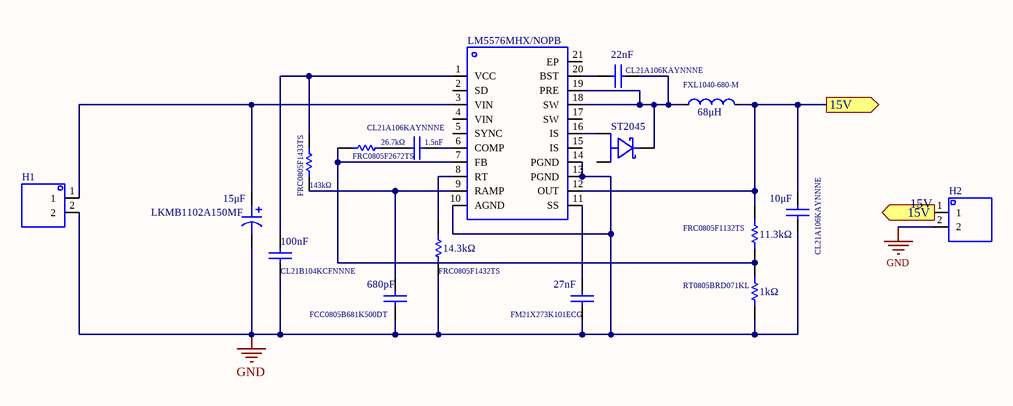
[diagram p0: MISC51833-3.schdoc]
# Altium project MISC51833-2.PrjPcb
1 sheet, 17 parts. Net scope: flat (ports and power ports of the same name join across sheets).
Board file: MISC51833.pcbdoc

## Sheet MISC51833-3.schdoc
size 292 x 193 mm; Name: MISC51833

### Parts
15μF  LKMB1102A150MF  [CAP-TH_BD5.0-P2.00-D0.8-FD]
C1  CL21A106KAYNNNE  value 1.5nF  [C0805]
C2  CL21A106KAYNNNE  value 22nF  [C0805]
C3  CL21A106KAYNNNE  value 10μF  [C0805]
C4  FCC0805B681K500DT  value 680pF  [C0805]
C5  FM21X273K101ECG  value 27nF  [C0805]
FRC0805F1132TS  value 11.3kΩ  [R0805]
FRC0805F1432TS  value 14.3kΩ  [R0805]
FRC0805F1433TS  value 143kΩ  [R0805]
FRC0805F2672TS  value 26.7kΩ  [R0805]
FXL1040-680-M  68μH  [IND-SMD_L11.5-W10.0_104CDMCCDS]
H1  (no value)  [HDR-TH_2P-P2.54-V-M-1]
H2  (no value)  [HDR-TH_2P-P2.54-V-M-1]
RT0805BRD071KL  value 1kΩ  [R0805]
ST2045  ST2045  [TO-277_3P-L5.4-W4.0-LS6.5-BR]  (value not drawn)
U1  LM5576MHX/NOPB  [HTSSOP-20_L6.5-W4.4-P0.65-LS6.4-BL-EP3.0]
U2  CL21B104KCFNNNE  value 100nF  [C0805]

### Ports
15V (out)

### Nets
GND: 15μF.2 C3.2 C4.2 C5.2 FRC0805F1432TS.2 H1.2 H2.2 RT0805BRD071KL.2 U1.10(AGND) U1.13(PGND) U1.14(PGND) U2.2
15V: C3.1 FRC0805F1132TS.1 FXL1040-680-M.2 H2.1 U1.12(OUT) ; port 15V
Net15μF_1: 15μF.1 H1.1 U1.3(VIN)
NetC1_1: C1.1 U1.6(COMP)
NetC1_2: C1.2 FRC0805F2672TS.1
NetC2_1: C2.1 FXL1040-680-M.1 ST2045.2(K) U1.18(SW) U1.19(PRE)
NetC2_2: C2.2 U1.20(BST)
NetC4_1: C4.1 FRC0805F1433TS.2 U1.9(RAMP)
NetC5_1: C5.1 U1.11(SS)
NetFRC0805F1132TS_2: FRC0805F1132TS.2 FRC0805F2672TS.2 RT0805BRD071KL.1 U1.7(FB)
NetFRC0805F1432TS_1: FRC0805F1432TS.1 U1.8(RT)
NetFRC0805F1433TS_1: FRC0805F1433TS.1 U1.1(VCC) U2.1
NetST2045_3: ST2045.3(A) U1.16(IS)

Not connected (* = marked no-connect by the designer): ST2045 1(A); U1 2(SD) 4(VIN) 5(SYNC) 15(IS) 17(SW) 21(EP)

### Library data of the parts
15μF = LKMB1102A150MF: UniqueId: 478177cd8fa5b5b0; SymbolName: LKMD1602K470MF; AddInBom: yes; Device: LKMB1102A150MF; DesignItemID: LKMD1602K470MF
C1 = CL21A106KAYNNNE: Capacitor; SimulationGenericComponent: True; UniqueId: 2b0dbff75b6442fd; AddInBom: yes; Device: CL21A106KAYNNNE; DesignItemID: Capacitor; LibraryName: Simulation Generic Components; SymbolName: Capacitor
C2 = CL21A106KAYNNNE: Capacitor; SimulationGenericComponent: True; UniqueId: gge1; AddInBom: yes; Device: CL21A106KAYNNNE; DesignItemID: Capacitor; LibraryName: Simulation Generic Components; SymbolName: Capacitor
C3 = CL21A106KAYNNNE: Capacitor; SimulationGenericComponent: True; UniqueId: gge2; AddInBom: yes; Device: CL21A106KAYNNNE; DesignItemID: Capacitor; LibraryName: Simulation Generic Components; SymbolName: Capacitor
C4 = FCC0805B681K500DT: Capacitor; SimulationGenericComponent: True; UniqueId: gge3; AddInBom: yes; Device: FCC0805B681K500DT; DesignItemID: Capacitor; LibraryName: Simulation Generic Components; SymbolName: Capacitor
C5 = FM21X273K101ECG: Capacitor; SimulationGenericComponent: True; UniqueId: gge5; AddInBom: yes; Device: FM21X273K101ECG; DesignItemID: Capacitor; LibraryName: Simulation Generic Components; SymbolName: Capacitor
FRC0805F1132TS = FRC0805F1132TS: Resistor; TC1: 0; SimulationGenericComponent: True; UniqueId: 093217a01aa01e1e; AddInBom: yes; Device: FRC0805F1132TS; TC2: 0; DesignItemID: Resistor; LibraryName: Simulation Generic Components; SymbolName: Resistor
FRC0805F1432TS = FRC0805F1432TS: Resistor; TC1: 0; SimulationGenericComponent: True; UniqueId: 0341c870ddcdfe59; AddInBom: yes; Device: FRC0805F1432TS; TC2: 0; DesignItemID: Resistor; LibraryName: Simulation Generic Components; SymbolName: Resistor
FRC0805F1433TS = FRC0805F1433TS: Resistor; TC1: 0; SimulationGenericComponent: True; UniqueId: 4b4c2ae898a29c1b; AddInBom: yes; Device: FRC0805F1433TS; TC2: 0; DesignItemID: Resistor; LibraryName: Simulation Generic Components; SymbolName: Resistor
FRC0805F2672TS = FRC0805F2672TS: Resistor; TC1: 0; SimulationGenericComponent: True; UniqueId: cfcb8c194707b4bb; AddInBom: yes; Device: FRC0805F2672TS; TC2: 0; DesignItemID: Resistor; LibraryName: Simulation Generic Components; SymbolName: Resistor
FXL1040-680-M = 68μH: UniqueId: a513e17394a354a6; SymbolName: FXL1040-680-M; AddInBom: yes; Device: 68μH; DesignItemID: FXL1040-680-M
H1 H2 = HDR-M_2.54_1x2P: Symbol: 210S-1*2P L=11.6MMGold-plated black; ConvertToPcb: yes; ModelId: 79b2e9f2d70a4d68a1b7098f27c6d4c50819f05c4eef4c71ace90d822a990e87; ModelName: HDR-M-2.54_1x2; ModelTransform: 200,100,0,0,0,0,0,0,-118.11; Device: HDR-M_2.54_1x2P; AddInBom: yes; SupplierPart: C124375; Supplier Footprint: 插件; FootprintName: HDR-TH_2P-P2.54-V-M-1
RT0805BRD071KL = RT0805BRD071KL: Resistor; TC1: 0; SimulationGenericComponent: True; UniqueId: 21a0b738a2499407; AddInBom: yes; Device: RT0805BRD071KL; TC2: 0; DesignItemID: Resistor; LibraryName: Simulation Generic Components; SymbolName: Resistor
ST2045 = ST2045: UniqueId: 40ecbfd5834ad512; AddInBom: yes; Device: ST2045; DesignItemID: ST2045; SymbolName: ST2045
U1 = LM5576MHX/NOPB: UniqueId: d82791b94b7d50e3; AddInBom: yes; Device: LM5576MHX/NOPB; DesignItemID: LM5576MHX/NOPB; SymbolName: LM5576MHX/NOPB
U2 = CL21B104KCFNNNE: Capacitor; SimulationGenericComponent: True; UniqueId: gge4; AddInBom: yes; Device: CL21B104KCFNNNE; DesignItemID: Capacitor; LibraryName: Simulation Generic Components; SymbolName: Capacitor